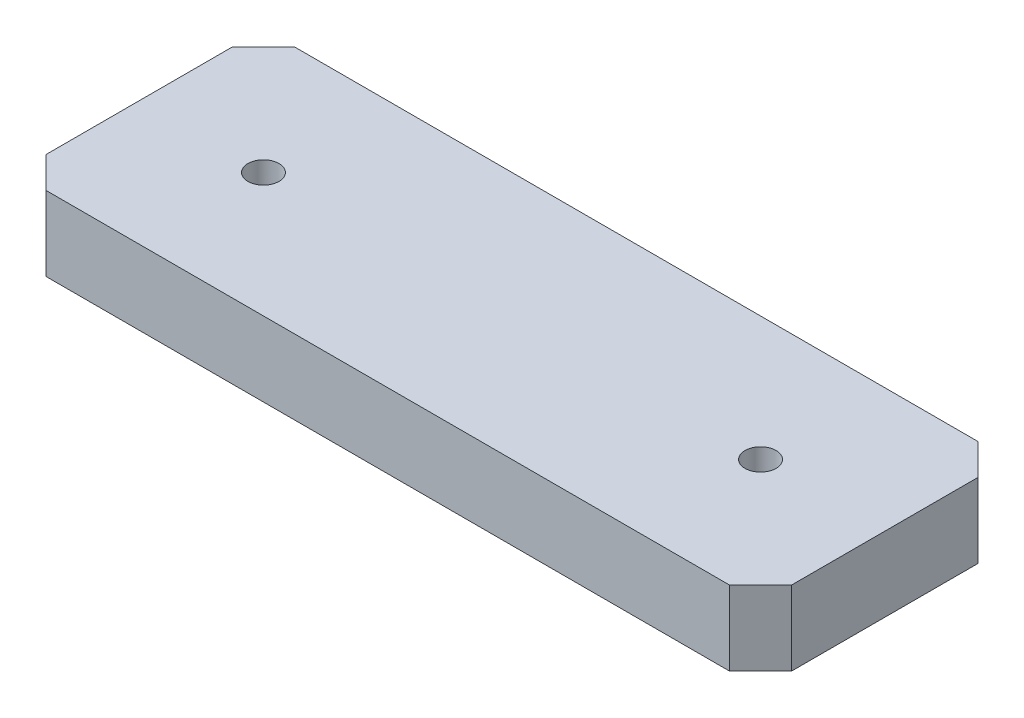
from build123d import *

# Parameters (mm, degrees)
SKETCH1_W             = 120
SKETCH1_H             = 40
EXTRUDE1_DEPTH        = 6
M6_TAPPED_HOLE1_D     = 5
M6_TAPPED_HOLE1_DEPTH = 15
M6_TAPPED_HOLE1_TIP   = 1.502151548
CHAMFER1_SIZE         = 5


with BuildPart() as part:
    # Sketch1 → Extrude1 (new, symmetric)
    with BuildSketch(Plane(origin=(0, 0, 0), x_dir=(1, 0, 0), z_dir=(0, 1, 0))):
        Rectangle(SKETCH1_W, SKETCH1_H)
    extrude(amount=EXTRUDE1_DEPTH, both=True)

    # M6 Tapped Hole1
    with Locations(Plane(origin=(0, 6, 0), x_dir=(-1, 0, 0), z_dir=(0, 1, 0))):
        with Locations((40, 0), (-40, 0)):
            Hole(M6_TAPPED_HOLE1_D / 2, depth=M6_TAPPED_HOLE1_DEPTH)
            with Locations((0, 0, -(M6_TAPPED_HOLE1_DEPTH + M6_TAPPED_HOLE1_TIP / 2))):  # 118° drill point
                Cone(0, M6_TAPPED_HOLE1_D / 2, M6_TAPPED_HOLE1_TIP, mode=Mode.SUBTRACT)

    # Chamfer1
    chamfer1_edges = [part.edges().sort_by_distance(p)[0] for p in [
        (-60, 0, -20),
        (60, 0, -20),
        (60, 0, 20),
        (-60, 0, 20),
    ]]
    chamfer(chamfer1_edges, length=CHAMFER1_SIZE)


solid = part.part
